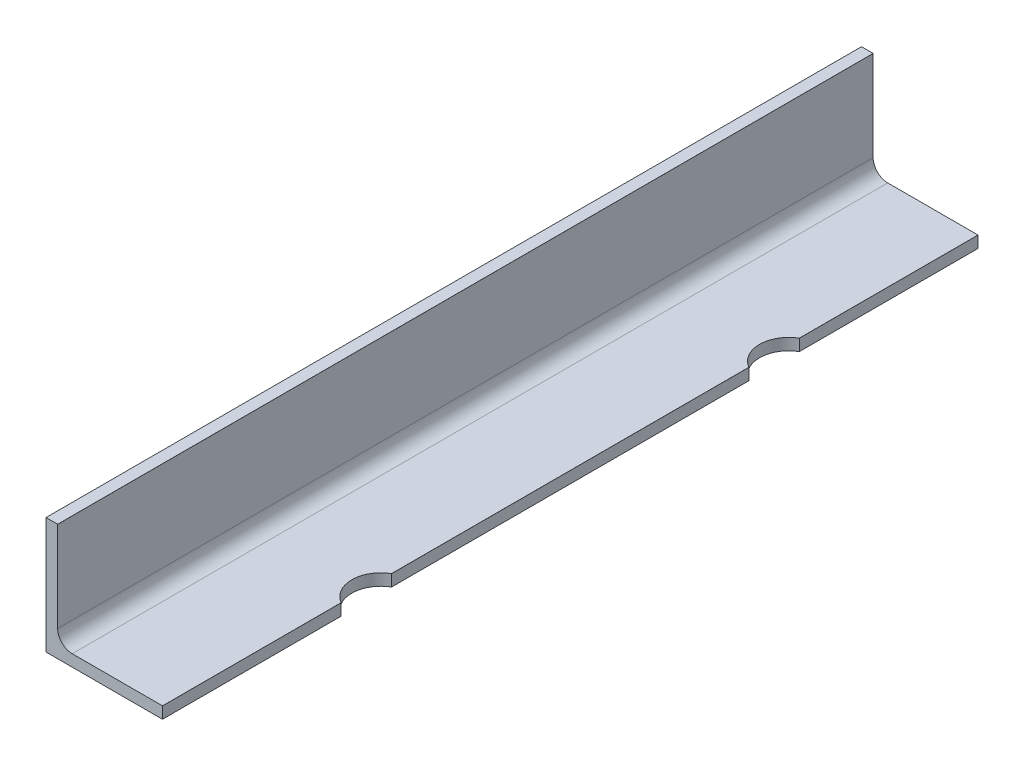
from build123d import *

# Parameters (mm, degrees)
EXTRUDE_1_DEPTH     = 280
SKETCH_2_R          = 10
CUT_EXTRUDE_1_DEPTH = 10


with BuildPart() as part:
    # 草图1 → 拉伸1 (new body)
    with BuildSketch(Plane.XY):
        with BuildLine():
            Line((0, 0), (0, 40))
            Line((0, 40), (3.99, 40))
            ThreePointArc((3.99, 40), (3.997071068, 39.997071068), (4, 39.99))
            Line((4, 39.99), (4, 9))
            ThreePointArc((4, 9), (5.464466094, 5.464466094), (9, 4))
            Line((9, 4), (39.99, 4))
            ThreePointArc((39.99, 4), (39.997071068, 3.997071068), (40, 3.99))
            Line((40, 3.99), (40, 0))
            Line((40, 0), (0, 0))
        make_face()
    extrude(amount=EXTRUDE_1_DEPTH)

    # 草图2 → 切除-拉伸1 (cut)
    with BuildSketch(Plane(origin=(0, 4, 0), x_dir=(1, 0, 0), z_dir=(0, 1, 0))):
        with Locations((45, -210)):
            Circle(SKETCH_2_R)
        with Locations((45, -70)):
            Circle(SKETCH_2_R)
    extrude(amount=-CUT_EXTRUDE_1_DEPTH, mode=Mode.SUBTRACT)


solid = part.part
